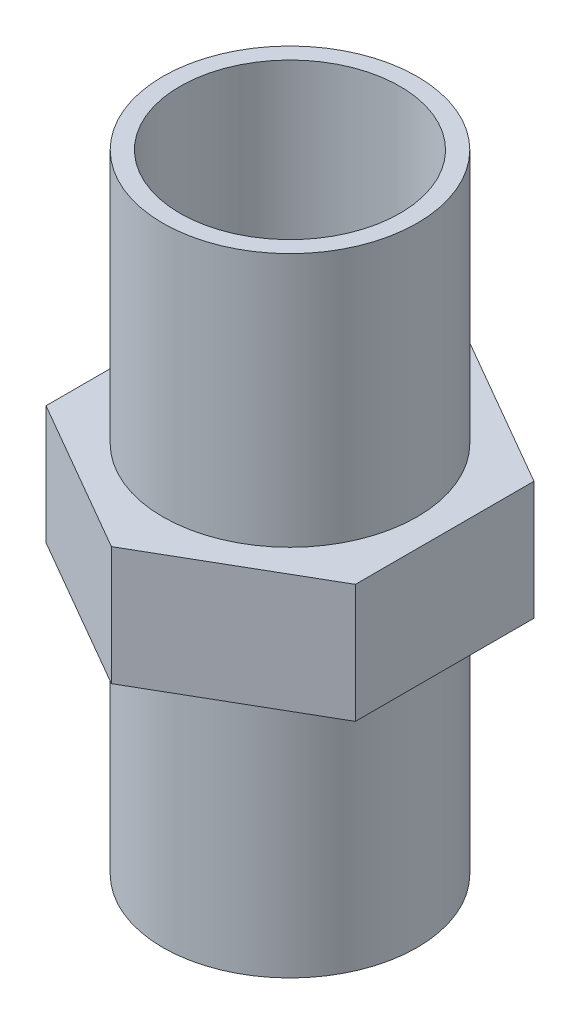
SolidWorks part; units mm, degrees
ref_plane "Front Plane" through (0, 0, 0) normal (0, 0, 1) x (1, 0, 0)
ref_plane "Top Plane" through (0, 0, 0) normal (0, 1, 0) x (1, 0, 0)
ref_plane "Right Plane" through (0, 0, 0) normal (1, 0, 0) x (0, 0, -1)
sketch "Sketch1" plane through (0, 0, 0) normal (0, 1, 0) x (1, 0, 0)
  circle A0 centre (0, 0) radius 7.5
  dimension "D1" = 15
extrude "Boss-Extrude1" add sketch "Sketch1" along normal blind 15
sketch "Sketch2" plane through (0, 15, 0) normal (0, 1, 0) x (1, 0, 0)
  line L1 (-9.123, 5.2672) -> (-9.123, -5.2672)
  line L2 (-9.123, -5.2672) -> (0, -10.5343)
  line L3 (0, -10.5343) -> (9.123, -5.2672)
  line L4 (9.123, -5.2672) -> (9.123, 5.2672)
  line L5 (9.123, 5.2672) -> (0, 10.5343)
  line L6 (0, 10.5343) -> (-9.123, 5.2672)
  circle A0 centre (0, 0) radius 9.123 construction
extrude "Boss-Extrude2" add sketch "Sketch2" along normal blind 7
sketch "Sketch3" plane through (0, 22, 0) normal (0, 1, 0) x (1, 0, 0)
  circle A1 centre (0, 0) radius 7.5
  circle A2 centre (0, 0) radius 7.5
  dimension "D1" = 0
extrude "Boss-Extrude3" add sketch "Sketch3" along normal blind 15
sketch "Sketch4" plane through (0, 37, 0) normal (0, 1, 0) x (1, 0, 0)
  circle A0 centre (0, 0) radius 6.489
extrude "Cut-Extrude1" cut sketch "Sketch4" against normal through all
